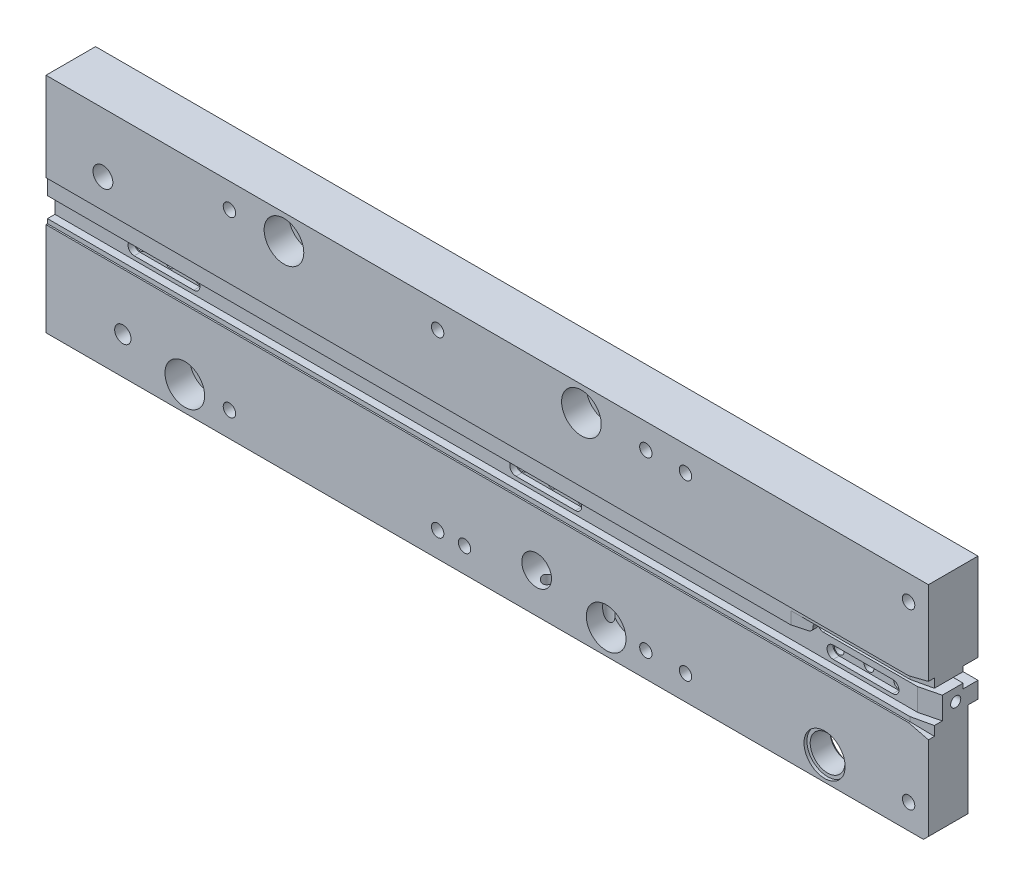
from build123d import *
from OCP.BRepFilletAPI import BRepFilletAPI_MakeChamfer

# Parameters (mm, degrees)
SKETCH1_W                                         = 350
SKETCH1_H                                         = 45
BOSS_EXTRUDE1_DEPTH                               = 10
CUT_EXTRUDE2_DEPTH                                = 0.3
CUT_EXTRUDE3_DEPTH                                = 1.8
CUT_EXTRUDE4_DEPTH                                = 177.72365433070925
CUT_EXTRUDE5_DEPTH                                = 3
CHAMFER1_SIZE                                     = 0.9
CHAMFER1_SIZE2                                    = 4
SKETCH7_W                                         = 55
SKETCH7_H                                         = 7.6
CUT_EXTRUDE6_DEPTH                                = 46.000000000000014
CUT_EXTRUDE7_DEPTH                                = 177.72365433070925
SKETCH9_W                                         = 49.99999999999999
SKETCH9_H                                         = 45
CUT_EXTRUDE8_DEPTH                                = 1.5
SKETCH10_R                                        = 2.249999999999996
SKETCH10_R_2                                      = 2.250000000000001
CUT_EXTRUDE9_DEPTH                                = 177.72365433070925
SKETCH11_R                                        = 4.000000000000006
SKETCH11_R_2                                      = 4
CUT_EXTRUDE10_DEPTH                               = 5
CUT_EXTRUDE11_START                               = -2.5
SKETCH12_R                                        = 4.000000000000006
SKETCH12_R_2                                      = 4.000000000000001
CUT_EXTRUDE11_DEPTH                               = 2.5
HOLE_SIZE_PER_HEX_BOLT_GRADE_C_TYPE_1_D           = 3.5
HOLE_SIZE_PER_HEX_BOLT_GRADE_C_TYPE_1_CBORE_D     = 6
HOLE_SIZE_PER_HEX_BOLT_GRADE_C_TYPE_1_CBORE_DEPTH = 5
SKETCH15_R                                        = 3.499999999999994
CUT_EXTRUDE12_DEPTH                               = 17.000000000000004
SKETCH19_W                                        = 24
SKETCH19_H                                        = 0.5000000000000346
CUT_EXTRUDE13_DEPTH                               = 6.999999999999998
CHAMFER2_SIZE                                     = 1
CHAMFER2_SIZE2                                    = 4
CHAMFER3_SIZE                                     = 4
CHAMFER3_SIZE2                                    = 1
CHAMFER4_SIZE                                     = 4
CHAMFER4_SIZE2                                    = 0.5
CUT_EXTRUDE14_REACH                               = 178.894
FILLET1_R                                         = 1
FILLET6_R                                         = 1
CUT_EXTRUDE15_DEPTH                               = 20
M3_TAPPED_HOLE2_D                                 = 2.5
M3_TAPPED_HOLE2_DEPTH                             = 7.5
M3_TAPPED_HOLE2_TIP                               = 0.7510757737844503
SKETCH30_R                                        = 3.999999999999999
SKETCH30_R_2                                      = 4.000000000000005
CUT_EXTRUDE20_DEPTH                               = 5
SKETCH31_R                                        = 2.2500000000000027
SKETCH31_R_2                                      = 2.2499999999999987
SKETCH31_R_3                                      = 2.2499999999999964
CUT_EXTRUDE21_DEPTH                               = 25.000000000000007
SKETCH32_W                                        = 54.999999999999986
SKETCH32_H                                        = 3
CUT_EXTRUDE22_DEPTH                               = 8
SKETCH33_R                                        = 3.9999999999999925
SKETCH33_R_2                                      = 4.000000000000005
CUT_EXTRUDE23_DEPTH                               = 5
SKETCH34_R                                        = 2.2500000000000093
SKETCH34_R_2                                      = 2.2499999999999964
CUT_EXTRUDE24_DEPTH                               = 19.000000000000004
SKETCH35_W                                        = 8
SKETCH35_H                                        = 8.000000000000007
CUT_EXTRUDE25_DEPTH                               = 5
M4_TAPPED_HOLE2_D                                 = 3.3
M4_TAPPED_HOLE2_DEPTH                             = 10.1
M4_TAPPED_HOLE2_TIP                               = 0.9914200213954745
SKETCH37_R                                        = 1.9999999999999996
CUT_EXTRUDE26_DEPTH                               = 6
CHAMFER5_SIZE                                     = 0.5
CHAMFER5_SIZE2                                    = 5
CHAMFER6_SIZE                                     = 5
CHAMFER6_SIZE2                                    = 0.5
FILLET8_R                                         = 1
M3_TAPPED_HOLE3_D                                 = 2.5
M3_TAPPED_HOLE3_DEPTH                             = 7.5
M3_TAPPED_HOLE3_TIP                               = 0.7510757737844503
CUT_EXTRUDE28_DEPTH                               = 3
SKETCH45_R                                        = 0.9999999999999983
SKETCH45_R_2                                      = 1.0000000000000016
CUT_EXTRUDE29_DEPTH                               = 5
SKETCH46_R                                        = 1.0000000000000002
CUT_EXTRUDE30_DEPTH                               = 50
SKETCH48_R                                        = 1.0000000000000016
SKETCH48_R_2                                      = 0.9999999999999983
CUT_EXTRUDE32_DEPTH                               = 177.72365433070925
CUT_EXTRUDE33_DEPTH                               = 2.5
SKETCH50_W                                        = 70.00000000000001
SKETCH50_H                                        = 26.641464115410763
CUT_EXTRUDE34_DEPTH                               = 60.00000000000003
SKETCH52_R                                        = 2.4999999999999796
CUT_EXTRUDE35_DEPTH                               = 10
M2_5_TAPPED_HOLE1_AT_2_COUNT                      = 2
M2_5_TAPPED_HOLE1_AT_2_PITCH                      = 8
SKETCH59_R                                        = 1.9999999999999967
CUT_EXTRUDE36_DEPTH                               = 5.5
FILLET9_R                                         = 3
FILLET10_R                                        = 1.5
CUT_EXTRUDE38_DEPTH                               = 96.00000000000003
CUT_EXTRUDE39_DEPTH                               = 2.8
SKETCH63_R                                        = 4.1499999999999835
CUT_EXTRUDE40_DEPTH                               = 0.6
SKETCH64_R                                        = 4.1499999999999835
CUT_EXTRUDE41_DEPTH                               = 0.6
FILLET11_R                                        = 1.5
M2_5_TAPPED_HOLE2_D                               = 2.05
M2_5_TAPPED_HOLE2_DEPTH                           = 5
M2_5_TAPPED_HOLE2_TIP                             = 0.6158821345032492
CHAMFER7_SIZE                                     = 1
BOSS_EXTRUDE2_DEPTH                               = 5.2


with BuildPart() as part:
    # Sketch1 → Boss-Extrude1 (new body)
    with BuildSketch(Plane.XY):
        Rectangle(SKETCH1_W, SKETCH1_H)
    extrude(amount=BOSS_EXTRUDE1_DEPTH)

    # Sketch3 → Cut-Extrude2 (cut)
    with BuildSketch(Plane.XY.offset(10)):
        Polygon((-175.00000000000003, 4.599999999999915), (174.99999999999997, 4.6), (174.99999999999997, -3.599999999999999), (-175.00000000000003, -3.599999999999999), align=None)
    extrude(amount=-CUT_EXTRUDE2_DEPTH, mode=Mode.SUBTRACT)

    # Sketch4 → Cut-Extrude3 (cut)
    with BuildSketch(Plane.XY.offset(10)):
        Polygon((174.99999999999997, 1.2999999999999654), (-175.00000000000003, 1.299999999999922), (-175.00000000000003, -2.7000000000000774), (174.99999999999997, -2.700000000000035), align=None)
    extrude(amount=-CUT_EXTRUDE3_DEPTH, mode=Mode.SUBTRACT)

    # Sketch5 → Cut-Extrude4 (cut, through all)
    with BuildSketch(Plane.XY.offset(10)):
        Polygon((150.99999999999997, 3.799999999999994), (174.99999999999997, 3.8), (174.99999999999997, 1.8), (150.99999999999997, 1.8), align=None)
    extrude(amount=-CUT_EXTRUDE4_DEPTH, mode=Mode.SUBTRACT)

    # Sketch6 → Cut-Extrude5 (cut)
    with BuildSketch(Plane(origin=(0, 0, 0), x_dir=(-1, 0, 0), z_dir=(0, 0, -1))):
        Polygon((-139.99999999999997, 0.8000000000000004), (-174.99999999999997, 0.7999999999999965), (-174.99999999999997, 4.799999999999997), (-139.99999999999997, 4.800000000000001), align=None)
    extrude(amount=-CUT_EXTRUDE5_DEPTH, mode=Mode.SUBTRACT)

    # Chamfer1: one chamfer whose edges measure the first distance from different faces: ONE call of the kernel's chamfer builder (chamfer() names one face for all edges)
    chamfer1_edges_1 = [part.edges().sort_by_distance(p)[0] for p in [
        (174.99999999999997, -3.1500000000000172, 9.7),
        (174.99999999999997, 1.5499999999999825, 9.7),
    ]]
    chamfer1_side_1 = [part.faces().sort_by_distance(p)[0] for p in [
        (174.99999999999997, -10.81544022721405, 4.909385489284791),
    ]]
    chamfer1_edges_2 = [part.edges().sort_by_distance(p)[0] for p in [
        (174.99999999999997, 4.199999999999999, 9.7),
    ]]
    chamfer1_side_2 = [part.faces().sort_by_distance(p)[0] for p in [
        (174.99999999999997, 13.306171092729647, 5.050805398345668),
    ]]
    chamfer1 = BRepFilletAPI_MakeChamfer(part.part.solid().wrapped)
    for e in chamfer1_edges_1:
        chamfer1.Add(CHAMFER1_SIZE, CHAMFER1_SIZE2, e.wrapped, chamfer1_side_1[0].wrapped)  # the first distance lies on this face
    for e in chamfer1_edges_2:
        chamfer1.Add(CHAMFER1_SIZE, CHAMFER1_SIZE2, e.wrapped, chamfer1_side_2[0].wrapped)  # the first distance lies on this face
    add(Compound.cast(chamfer1.Shape()), mode=Mode.REPLACE)

    # Sketch7 → Cut-Extrude6 (cut)
    with BuildSketch(Plane.XY.offset(10)):
        with Locations((-113, 0.49999999999998157)):
            Rectangle(SKETCH7_W, SKETCH7_H)
    extrude(amount=-CUT_EXTRUDE6_DEPTH, mode=Mode.SUBTRACT)

    # Sketch8 → Cut-Extrude7 (cut, through all)
    with BuildSketch(Plane.XY.offset(10)):
        Polygon((-63.00000000000003, 9.5), (-13.000000000000032, 9.5), (-13.000000000000028, -8.499999999999998), (-63.00000000000003, -8.499999999999998), align=None)
    extrude(amount=-CUT_EXTRUDE7_DEPTH, mode=Mode.SUBTRACT)

    # Sketch9 → Cut-Extrude8 (cut)
    with BuildSketch(Plane.XY.offset(10)):
        with Locations((-38.000000000000036, 0)):
            Rectangle(SKETCH9_W, SKETCH9_H)
    extrude(amount=-CUT_EXTRUDE8_DEPTH, mode=Mode.SUBTRACT)

    # Sketch10 → Cut-Extrude9 (cut, through all)
    with BuildSketch(Plane.XY.offset(10)):
        with Locations((-69, 11.49999999999999)):
            Circle(SKETCH10_R)
        with Locations((-69.00000000000001, -10.500000000000007)):
            Circle(SKETCH10_R)
        with Locations((-7.000000000000017, -10.500000000000018)):
            Circle(SKETCH10_R_2)
        with Locations((-7.00000000000001, 11.499999999999979)):
            Circle(SKETCH10_R_2)
    extrude(amount=-CUT_EXTRUDE9_DEPTH, mode=Mode.SUBTRACT)

    # Sketch11 → Cut-Extrude10 (cut)
    with BuildSketch(Plane.XY.offset(10)):
        with Locations((-69, 11.49999999999999)):
            Circle(SKETCH11_R)
        with Locations((-69.00000000000001, -10.500000000000007)):
            Circle(SKETCH11_R)
        with Locations((-7.000000000000017, -10.500000000000018)):
            Circle(SKETCH11_R_2)
        with Locations((-7.00000000000001, 11.499999999999979)):
            Circle(SKETCH11_R_2)
    extrude(amount=-CUT_EXTRUDE10_DEPTH, mode=Mode.SUBTRACT)

    # Sketch12 → Cut-Extrude11 (cut)
    with BuildSketch(Plane(origin=(0, 0, 0), x_dir=(-1, 0, 0), z_dir=(0, 0, -1)).offset(CUT_EXTRUDE11_START)):
        with Locations(Location((69, 11.49999999999999, 0), (0, 0, 180))):
            Circle(SKETCH12_R)
        with Locations(Location((7.000000000000017, -10.500000000000018, 0), (0, 0, 180))):
            Circle(SKETCH12_R_2)
    extrude(amount=CUT_EXTRUDE11_DEPTH, mode=Mode.SUBTRACT)

    # Hole size per hex bolt grade C type 1 (through all)
    with Locations(Plane(origin=(95.97, -14.5, 10), x_dir=(1, 0, 0), z_dir=(0, 0, 1))):
        with Locations((0, 0)):
            CounterBoreHole(HOLE_SIZE_PER_HEX_BOLT_GRADE_C_TYPE_1_D / 2, HOLE_SIZE_PER_HEX_BOLT_GRADE_C_TYPE_1_CBORE_D / 2, HOLE_SIZE_PER_HEX_BOLT_GRADE_C_TYPE_1_CBORE_DEPTH)

    # Sketch15 → Cut-Extrude12 (cut)
    with BuildSketch(Plane.XY.offset(10)):
        with Locations((154.04999999999995, -17.669999999999998)):
            Circle(SKETCH15_R)
    extrude(amount=-CUT_EXTRUDE12_DEPTH, mode=Mode.SUBTRACT)

    # Sketch19 → Cut-Extrude13 (cut)
    with BuildSketch(Plane.XY.offset(8.200000000000001)):
        with Locations((162.99999999999997, 1.5499999999999827)):
            Rectangle(SKETCH19_W, SKETCH19_H)
    extrude(amount=CUT_EXTRUDE13_DEPTH, mode=Mode.SUBTRACT)

    # Chamfer2: one chamfer whose edges measure the first distance from different faces: ONE call of the kernel's chamfer builder (chamfer() names one face for all edges)
    chamfer2_edges_1 = [part.edges().sort_by_distance(p)[0] for p in [
        (174.99999999999997, -0.4500000000000173, 8.2),
    ]]
    chamfer2_side_1 = [part.faces().sort_by_distance(p)[0] for p in [
        (174.99999999999997, -10.882518845853916, 4.88102417468157),
    ]]
    chamfer2_edges_2 = [part.edges().sort_by_distance(p)[0] for p in [
        (174.99999999999997, 4.6, 9.399999999999999),
    ]]
    chamfer2_side_2 = [part.faces().sort_by_distance(p)[0] for p in [
        (174.99999999999997, 13.341990821678323, 5.034287587412589),
    ]]
    chamfer2 = BRepFilletAPI_MakeChamfer(part.part.solid().wrapped)
    for e in chamfer2_edges_1:
        chamfer2.Add(CHAMFER2_SIZE, CHAMFER2_SIZE2, e.wrapped, chamfer2_side_1[0].wrapped)  # the first distance lies on this face
    for e in chamfer2_edges_2:
        chamfer2.Add(CHAMFER2_SIZE, CHAMFER2_SIZE2, e.wrapped, chamfer2_side_2[0].wrapped)  # the first distance lies on this face
    add(Compound.cast(chamfer2.Shape()), mode=Mode.REPLACE)

    # Chamfer3
    chamfer3_edges = [part.edges().sort_by_distance(p)[0] for p in [
        (174.99999999999997, -3.599999999999999, 9.399999999999999),
    ]]
    chamfer3_side = [part.faces().sort_by_distance(p)[0] for p in [
        (83.86597938144327, -3.599999999999999, 9.836082474226805),
    ]]
    chamfer(chamfer3_edges, length=CHAMFER3_SIZE, length2=CHAMFER3_SIZE2, reference=chamfer3_side[0])

    # Chamfer4
    chamfer4_edges = [part.edges().sort_by_distance(p)[0] for p in [
        (150.99999999999997, 1.2999999999999654, 8.95),
    ]]
    chamfer4_side = [part.faces().sort_by_distance(p)[0] for p in [
        (68.99999999999997, 1.2999999999999523, 8.95),
    ]]
    chamfer(chamfer4_edges, length=CHAMFER4_SIZE, length2=CHAMFER4_SIZE2, reference=chamfer4_side[0])

    # Cut-Extrude14: up to this face of the body (flat: up to its plane)
    cut_extrude14_end = Plane(part.part.faces().sort_by_distance((162.879245283, 3.8, 6.315471698))[0])
    # Sketch21 → Cut-Extrude14 (cut, up to the picked face)
    with BuildSketch(Plane.XZ.offset(-1.2999999999999439), mode=Mode.PRIVATE) as cut_extrude14_sk1:
        Polygon((146.99999999999986, 9.700000000000001), (151.5522483304892, 9.700000000000001), (151.5522483304892, 9.2), align=None)
    cut_extrude14_tool1 = split(extrude(cut_extrude14_sk1.sketch, amount=-CUT_EXTRUDE14_REACH, mode=Mode.PRIVATE), bisect_by=cut_extrude14_end, keep=Keep.BOTH, mode=Mode.PRIVATE)
    add(cut_extrude14_tool1.solids().sort_by(Axis((150.034832, 1.3, 9.533333), (-1.2e-16, 1, 0)))[0], mode=Mode.SUBTRACT)

    # Fillet1
    fillet1_edges = [part.edges().sort_by_distance(p)[0] for p in [
        (150.99999999999997, 3.799999999999994, 6.1303283284652155),
    ]]
    fillet(fillet1_edges, radius=FILLET1_R)

    # Fillet6
    fillet6_edges = [part.edges().sort_by_distance(p)[0] for p in [
        (150.99999999999997, 1.7999999999999625, 8.730328328465212),
    ]]
    fillet(fillet6_edges, radius=FILLET6_R)

    # Sketch22 → Cut-Extrude15 (cut)
    with BuildSketch(Plane.XZ.offset(22.5)):
        Polygon((174.99999999999997, 0), (139.99999999999997, -4.29e-15), (139.99999999999997, 1.9999999999999958), (174.99999999999997, 2), align=None)
    extrude(amount=-CUT_EXTRUDE15_DEPTH, mode=Mode.SUBTRACT)

    # M3 Tapped Hole2
    with Locations(Plane.XY.offset(10)):
        with Locations((34, -17.5), (34, 17.5), (76, -17.5), (76, 17.5), (118, -17.5), (118, 17.5), (126, 17.5), (126, -17.5), (171, -17.5), (171, 17.5)):
            Hole(M3_TAPPED_HOLE2_D / 2, depth=M3_TAPPED_HOLE2_DEPTH)
            with Locations((0, 0, -(M3_TAPPED_HOLE2_DEPTH + M3_TAPPED_HOLE2_TIP / 2))):  # 118° drill point
                Cone(0, M3_TAPPED_HOLE2_D / 2, M3_TAPPED_HOLE2_TIP, mode=Mode.SUBTRACT)

    # Sketch30 → Cut-Extrude20 (cut)
    with BuildSketch(Plane.XY.offset(10)):
        with Locations((24.99999999999994, -17.499999999999996)):
            Circle(SKETCH30_R)
        with Locations((109.99999999999994, -17.499999999999996)):
            Circle(SKETCH30_R_2)
        with Locations((104.99999999999996, 17.499999999999996)):
            Circle(SKETCH30_R_2)
        with Locations((44.99999999999996, 17.499999999999996)):
            Circle(SKETCH30_R_2)
    extrude(amount=-CUT_EXTRUDE20_DEPTH, mode=Mode.SUBTRACT)

    # Sketch31 → Cut-Extrude21 (cut)
    with BuildSketch(Plane.XY.offset(10)):
        with Locations((44.99999999999996, 17.499999999999996)):
            Circle(SKETCH31_R)
        with Locations((24.99999999999994, -17.499999999999996)):
            Circle(SKETCH31_R_2)
        with Locations((109.99999999999994, -17.499999999999996)):
            Circle(SKETCH31_R_3)
        with Locations((104.99999999999996, 17.499999999999996)):
            Circle(SKETCH31_R_3)
    extrude(amount=-CUT_EXTRUDE21_DEPTH, mode=Mode.SUBTRACT)

    # Sketch32 → Cut-Extrude22 (cut)
    with BuildSketch(Plane.XZ.offset(22.5)):
        with Locations((-105.5, 1.5)):
            Rectangle(SKETCH32_W, SKETCH32_H)
    extrude(amount=-CUT_EXTRUDE22_DEPTH, mode=Mode.SUBTRACT)

    # Sketch33 → Cut-Extrude23 (cut)
    with BuildSketch(Plane.XY.offset(10)):
        with Locations((-160.00000000000003, 17.499999999999996)):
            Circle(SKETCH33_R)
        with Locations((-95.00000000000003, 17.499999999999996)):
            Circle(SKETCH33_R_2)
        with Locations((-160.00000000000003, -17.499999999999996)):
            Circle(SKETCH33_R)
    extrude(amount=-CUT_EXTRUDE23_DEPTH, mode=Mode.SUBTRACT)

    # Sketch34 → Cut-Extrude24 (cut)
    with BuildSketch(Plane.XY.offset(10)):
        with Locations((-160.00000000000003, 17.499999999999996)):
            Circle(SKETCH34_R)
        with Locations((-160.00000000000003, -17.499999999999996)):
            Circle(SKETCH34_R)
        with Locations((-95.00000000000003, 17.499999999999996)):
            Circle(SKETCH34_R_2)
    extrude(amount=-CUT_EXTRUDE24_DEPTH, mode=Mode.SUBTRACT)

    # Sketch35 → Cut-Extrude25 (cut)
    with BuildSketch(Plane.XY.offset(10)):
        with Locations((-160.00000000000003, 21.5)):
            Rectangle(SKETCH35_W, SKETCH35_H)
        with Locations((-95.00000000000003, 21.5)):
            Rectangle(SKETCH35_W, SKETCH35_H)
        with Locations((-160.00000000000003, -21.5)):
            Rectangle(SKETCH35_W, SKETCH35_H)
    extrude(amount=-CUT_EXTRUDE25_DEPTH, mode=Mode.SUBTRACT)

    # M4 Tapped Hole2
    with Locations(Plane(origin=(12.5, -15, 10), x_dir=(1, 0, 0), z_dir=(0, 0, 1))):
        with Locations((0, 0)):
            Hole(M4_TAPPED_HOLE2_D / 2, depth=M4_TAPPED_HOLE2_DEPTH)
            with Locations((0, 0, -(M4_TAPPED_HOLE2_DEPTH + M4_TAPPED_HOLE2_TIP / 2))):  # 118° drill point
                Cone(0, M4_TAPPED_HOLE2_D / 2, M4_TAPPED_HOLE2_TIP, mode=Mode.SUBTRACT)

    # Sketch37 → Cut-Extrude26 (cut)
    with BuildSketch(Plane.XY.offset(10)):
        with Locations((8.47999999999996, 10.500000000000002)):
            Circle(SKETCH37_R)
    extrude(amount=-CUT_EXTRUDE26_DEPTH, mode=Mode.SUBTRACT)

    # Chamfer5: one chamfer whose edges measure the first distance from different faces: ONE call of the kernel's chamfer builder (chamfer() names one face for all edges)
    chamfer5_edges_1 = [part.edges().sort_by_distance(p)[0] for p in [
        (-140.5, -2.7000000000000735, 8.95),
        (-140.5, 1.299999999999926, 8.950000000000001),
    ]]
    chamfer5_side_1 = [part.faces().sort_by_distance(p)[0] for p in [
        (-140.5, 0.6063201417601755, 4.486739515652685),
    ]]
    chamfer5_edges_2 = [part.edges().sort_by_distance(p)[0] for p in [
        (-63.00000000000003, -3.5999999999999996, 9.85),
        (-63.00000000000003, -2.7000000000000637, 8.95),
        (-63.00000000000002, 1.2999999999999359, 8.95),
        (-63.00000000000003, 4.599999999999943, 9.85),
    ]]
    chamfer5_side_2 = [part.faces().sort_by_distance(p)[0] for p in [
        (-63.00000000000003, 0.3747877758913459, 5.643718166383701),
    ]]
    chamfer5 = BRepFilletAPI_MakeChamfer(part.part.solid().wrapped)
    for e in chamfer5_edges_1:
        chamfer5.Add(CHAMFER5_SIZE, CHAMFER5_SIZE2, e.wrapped, chamfer5_side_1[0].wrapped)  # the first distance lies on this face
    for e in chamfer5_edges_2:
        chamfer5.Add(CHAMFER5_SIZE, CHAMFER5_SIZE2, e.wrapped, chamfer5_side_2[0].wrapped)  # the first distance lies on this face
    add(Compound.cast(chamfer5.Shape()), mode=Mode.REPLACE)

    # Chamfer6: one chamfer whose edges measure the first distance from different faces: ONE call of the kernel's chamfer builder (chamfer() names one face for all edges)
    chamfer6_edges_1 = [part.edges().sort_by_distance(p)[0] for p in [
        (-63.00000000000003, -3.6500000000000314, 9.7),
        (-140.5, -3.2500000000000453, 9.7),
    ]]
    chamfer6_side_1 = [part.faces().sort_by_distance(p)[0] for p in [
        (-76.75000000000001, -2.812008749658295, 9.7),
    ]]
    chamfer6_edges_2 = [part.edges().sort_by_distance(p)[0] for p in [
        (-63.00000000000003, 3.449999999999939, 9.7),
        (-140.5, 3.0499999999999527, 9.7),
    ]]
    chamfer6_side_2 = [part.faces().sort_by_distance(p)[0] for p in [
        (-160.25, 2.420644457443943, 9.7),
    ]]
    chamfer6 = BRepFilletAPI_MakeChamfer(part.part.solid().wrapped)
    for e in chamfer6_edges_1:
        chamfer6.Add(CHAMFER6_SIZE, CHAMFER6_SIZE2, e.wrapped, chamfer6_side_1[0].wrapped)  # the first distance lies on this face
    for e in chamfer6_edges_2:
        chamfer6.Add(CHAMFER6_SIZE, CHAMFER6_SIZE2, e.wrapped, chamfer6_side_2[0].wrapped)  # the first distance lies on this face
    add(Compound.cast(chamfer6.Shape()), mode=Mode.REPLACE)

    # Fillet8
    fillet8_edges = [part.edges().sort_by_distance(p)[0] for p in [
        (-85.5, -3.3000000000000185, 4.85),
        (-85.5, 4.299999999999981, 4.85),
        (-140.5, -3.3000000000000185, 4.6),
        (-140.5, 4.299999999999981, 4.6),
    ]]
    fillet(fillet8_edges, radius=FILLET8_R)

    # M3 Tapped Hole3
    with Locations(Plane.XY.offset(8.5)):
        with Locations((-57, -16), (-19, -16), (-19, 17), (-57, 17)):
            Hole(M3_TAPPED_HOLE3_D / 2, depth=M3_TAPPED_HOLE3_DEPTH)
            with Locations((0, 0, -(M3_TAPPED_HOLE3_DEPTH + M3_TAPPED_HOLE3_TIP / 2))):  # 118° drill point
                Cone(0, M3_TAPPED_HOLE3_D / 2, M3_TAPPED_HOLE3_TIP, mode=Mode.SUBTRACT)

    # Sketch44 → Cut-Extrude28 (cut)
    with BuildSketch(Plane.XY.offset(10)):
        with BuildLine():
            Line((165.99999999999994, -1.9500000000000404), (153.99999999999994, -1.9500000000000417))
            ThreePointArc((153.99999999999994, -1.9500000000000417), (152.74999999999994, -0.7000000000000418), (153.99999999999994, 0.5499999999999583))
            Line((153.99999999999994, 0.5499999999999583), (165.99999999999994, 0.5499999999999601))
            ThreePointArc((165.99999999999994, 0.5499999999999601), (167.24999999999994, -0.7000000000000408), (165.99999999999994, -1.9500000000000404))
        make_face()
        with BuildLine():
            Line((101.99999999999997, -1.950000000000045), (89.99999999999997, -1.9500000000000468))
            ThreePointArc((89.99999999999997, -1.9500000000000468), (88.74999999999997, -0.700000000000047), (89.99999999999997, 0.5499999999999524))
            Line((89.99999999999997, 0.5499999999999524), (101.99999999999997, 0.5499999999999537))
            ThreePointArc((101.99999999999997, 0.5499999999999537), (103.24999999999997, -0.7000000000000444), (101.99999999999997, -1.950000000000045))
        make_face()
        with BuildLine():
            Line((12.999999999999966, 0.5499999999999424), (24.999999999999968, 0.5499999999999424))
            ThreePointArc((24.999999999999968, 0.5499999999999424), (26.249999999999964, -0.7000000000000582), (24.999999999999968, -1.950000000000056))
            Line((24.999999999999968, -1.950000000000056), (12.999999999999966, -1.950000000000056))
            ThreePointArc((12.999999999999966, -1.950000000000056), (11.749999999999966, -0.700000000000057), (12.999999999999966, 0.5499999999999424))
        make_face()
    extrude(amount=-CUT_EXTRUDE28_DEPTH, mode=Mode.SUBTRACT)

    # Sketch45 → Cut-Extrude29 (cut)
    with BuildSketch(Plane.XY.offset(10)):
        with Locations((165.99999999999994, -0.7000000000000408)):
            Circle(SKETCH45_R)
        with Locations((153.99999999999994, -0.7000000000000419)):
            Circle(SKETCH45_R)
        with Locations((101.99999999999997, -0.7000000000000444)):
            Circle(SKETCH45_R)
        with Locations((89.99999999999997, -0.7000000000000471)):
            Circle(SKETCH45_R)
        with Locations((24.999999999999968, -0.7000000000000582)):
            Circle(SKETCH45_R_2)
        with Locations((12.999999999999966, -0.7000000000000571)):
            Circle(SKETCH45_R_2)
        with Locations((159.99999999999994, -0.7000000000000413)):
            Circle(SKETCH45_R)
        with Locations((96.0000000000018, -0.6999999999974267)):
            Circle(SKETCH45_R)
        with Locations((18.999999999988503, -0.6999999999974267)):
            Circle(SKETCH45_R_2)
    extrude(amount=-CUT_EXTRUDE29_DEPTH, mode=Mode.SUBTRACT)

    # Sketch46 → Cut-Extrude30 (cut)
    with BuildSketch(Plane(origin=(174.99999999999997, 0, 0), x_dir=(0, 0, -1), z_dir=(1, 0, 0))):
        with Locations((-4.5, -0.6999999999999993)):
            Circle(SKETCH46_R)
    extrude(amount=-CUT_EXTRUDE30_DEPTH, mode=Mode.SUBTRACT)

    # Sketch48 → Cut-Extrude32 (cut, through all)
    with BuildSketch(Plane.XY.offset(10)):
        with Locations((12.999999999999966, -0.7000000000000571)):
            Circle(SKETCH48_R)
        with Locations((18.999999999988503, -0.6999999999974267)):
            Circle(SKETCH48_R)
        with Locations((24.999999999999968, -0.7000000000000582)):
            Circle(SKETCH48_R)
        with Locations((101.99999999999997, -0.7000000000000444)):
            Circle(SKETCH48_R_2)
        with Locations((96.0000000000018, -0.6999999999974267)):
            Circle(SKETCH48_R_2)
        with Locations((89.99999999999997, -0.7000000000000471)):
            Circle(SKETCH48_R_2)
    extrude(amount=-CUT_EXTRUDE32_DEPTH, mode=Mode.SUBTRACT)

    # Sketch49 → Cut-Extrude33 (cut)
    with BuildSketch(Plane(origin=(0, 0, 0), x_dir=(-1, 0, 0), z_dir=(0, 0, -1))):
        with BuildLine():
            Line((-103.50000000000182, 1.3000000000025718), (-88.50000000000182, 1.3000000000025707))
            ThreePointArc((-88.50000000000182, 1.3000000000025707), (-86.5000000000018, -0.6999999999974215), (-88.5000000000018, -2.699999999997429))
            Line((-88.5000000000018, -2.699999999997429), (-103.50000000000182, -2.699999999997429))
            ThreePointArc((-103.50000000000182, -2.699999999997429), (-105.50000000000182, -0.6999999999974283), (-103.50000000000182, 1.3000000000025718))
        make_face()
        with BuildLine():
            Line((-26.499999999988507, 1.3000000000025913), (-11.499999999988495, 1.3000000000025913))
            ThreePointArc((-11.499999999988495, 1.3000000000025913), (-9.499999999988496, -0.6999999999974087), (-11.499999999988495, -2.6999999999974076))
            Line((-11.499999999988495, -2.6999999999974076), (-26.499999999988507, -2.6999999999974076))
            ThreePointArc((-26.499999999988507, -2.6999999999974076), (-28.499999999988507, -0.6999999999974085), (-26.499999999988507, 1.3000000000025913))
        make_face()
    extrude(amount=-CUT_EXTRUDE33_DEPTH, mode=Mode.SUBTRACT)

    # Sketch50 → Cut-Extrude34 (cut)
    with BuildSketch(Plane(origin=(0, 22.5, 0), x_dir=(1, 0, 0), z_dir=(0, 1, 0))):
        with Locations((-38.000000000000036, 0)):
            Rectangle(SKETCH50_W, SKETCH50_H)
    extrude(amount=-CUT_EXTRUDE34_DEPTH, mode=Mode.SUBTRACT)


with BuildPart() as cut_extrude34_piece_1:
    # of the separate pieces the step leaves, piece 1, a body of its own (cut_extrude34_pieces)
    add(part.part.solids().sort_by_distance((-3, 22.5, 0))[0])

    # Sketch51 → M3 Tapped Hole4 (revolve, cut)
    with BuildSketch(Plane(origin=(95.96999999999996, -22.5, 7.5), x_dir=(0, 0, -1), z_dir=(1, 0, 0))):
        Polygon((0, 0), (-2.02e-15, 8.25107577378445), (1.2499999999999976, 7.5), (1.2499999999999987, -5e-17), align=None)
    revolve(axis=Axis((95.96999999999996, -28.84999999999999, 7.5), (0, 1, 0)), mode=Mode.SUBTRACT)

    # Sketch52 → Cut-Extrude35 (cut)
    with BuildSketch(Plane.XZ.offset(22.5)):
        with Locations(Location((81.41999999999996, 3.999999999999949, 0), (0, 0, 270))):
            Circle(SKETCH52_R)
    extrude(amount=-CUT_EXTRUDE35_DEPTH, mode=Mode.SUBTRACT)

    # Sketch53 → M3 Tapped Hole5 (revolve, cut)
    with BuildSketch(Plane(origin=(81.41999999999996, -17.499999999999996, 10), x_dir=(0, -1, 0), z_dir=(1, 0, 0))):
        Polygon((0, 0), (-2.02e-15, 8.251075773784452), (1.2499999999999871, 7.499999999999993), (1.249999999999989, -1.4e-15), align=None)
    revolve(axis=Axis((81.41999999999996, -17.499999999999996, 16.34999999999999), (0, 0, -1)), mode=Mode.SUBTRACT)

    # Sketch55 → M2.5 Tapped Hole1 (revolve, cut)
    with BuildSketch(Plane(origin=(113.99999999999996, -22.5, 5.7), x_dir=(0, 0, -1), z_dir=(1, 0, 0))):
        Polygon((0, 0), (-1.71e-15, 6.965882134503248), (1.0249999999999984, 6.35), (1.024999999999999, -3e-17), align=None)
    m2_5_tapped_hole1 = revolve(axis=Axis((113.99999999999996, -28.84999999999999, 5.7), (0, 1, 0)), mode=Mode.SUBTRACT)

    # M2.5 Tapped Hole1 at 2: M2.5 Tapped Hole1 ×2
    with Locations(*[(-i * M2_5_TAPPED_HOLE1_AT_2_PITCH, 0, 0) for i in range(1, M2_5_TAPPED_HOLE1_AT_2_COUNT)]):
        add(m2_5_tapped_hole1, mode=Mode.SUBTRACT)

    # Sketch59 → Cut-Extrude36 (cut)
    with BuildSketch(Plane(origin=(0, 0, 0), x_dir=(-1, 0, 0), z_dir=(0, 0, -1))):
        with Locations((-124.99999999999996, -0.6999999999999993)):
            Circle(SKETCH59_R)
    extrude(amount=-CUT_EXTRUDE36_DEPTH, mode=Mode.SUBTRACT)

    # Fillet9
    fillet9_edges = [cut_extrude34_piece_1.edges().sort_by_distance(p)[0] for p in [
        (139.99999999999997, -2.5, 0.9999999999999957),
    ]]
    fillet(fillet9_edges, radius=FILLET9_R)

    # Fillet10
    fillet10_edges = [cut_extrude34_piece_1.edges().sort_by_distance(p)[0] for p in [
        (139.99999999999997, 4.800000000000001, 1.5),
        (139.99999999999997, 0.8000000000000004, 1.5),
    ]]
    fillet(fillet10_edges, radius=FILLET10_R)

    # Sketch62 → Cut-Extrude39 (cut)
    with BuildSketch(Plane(origin=(-2.5e-16, 0, 1.9999999999999785), x_dir=(-1, 0, -1.2e-16), z_dir=(1.2e-16, 0, -1))):
        Polygon((-164.04999999999998, -30.002737548386204), (-144.04999999999995, -30.0027375483862), (-144.04999999999995, -10), (-164.04999999999998, -10.000000000000002), align=None)
    extrude(amount=-CUT_EXTRUDE39_DEPTH, mode=Mode.SUBTRACT)

    # Sketch63 → Cut-Extrude40 (cut)
    with BuildSketch(Plane.XY.offset(10)):
        with Locations((154.04999999999995, -17.669999999999998)):
            Circle(SKETCH63_R)
    extrude(amount=-CUT_EXTRUDE40_DEPTH, mode=Mode.SUBTRACT)

    # Sketch64 → Cut-Extrude41 (cut)
    with BuildSketch(Plane(origin=(-6.2e-16, 0, 4.799999999999978), x_dir=(-1, 0, -1.3e-16), z_dir=(1.3e-16, 0, -1))):
        with Locations(Location((-154.04999999999995, -17.669999999999998, 0), (0, 0, 180))):
            Circle(SKETCH64_R)
    extrude(amount=-CUT_EXTRUDE41_DEPTH, mode=Mode.SUBTRACT)

    # Fillet11
    fillet11_edges = [cut_extrude34_piece_1.edges().sort_by_distance(p)[0] for p in [
        (144.04999999999995, -10, 3.399999999999996),
        (164.04999999999998, -10.000000000000002, 3.3999999999999986),
    ]]
    fillet(fillet11_edges, radius=FILLET11_R)

    # M2.5 Tapped Hole2
    with Locations(Plane(origin=(175, -0.7, 4.5), x_dir=(0, 0, 1), z_dir=(1, 0, 0))):
        with Locations((0, 0)):
            Hole(M2_5_TAPPED_HOLE2_D / 2, depth=M2_5_TAPPED_HOLE2_DEPTH)
            with Locations((0, 0, -(M2_5_TAPPED_HOLE2_DEPTH + M2_5_TAPPED_HOLE2_TIP / 2))):  # 118° drill point
                Cone(0, M2_5_TAPPED_HOLE2_D / 2, M2_5_TAPPED_HOLE2_TIP, mode=Mode.SUBTRACT)

    # Chamfer7
    chamfer7_edges = [cut_extrude34_piece_1.edges().sort_by_distance(p)[0] for p in [
        (174.99999999999997, -22.5, 6),
    ]]
    chamfer(chamfer7_edges, length=CHAMFER7_SIZE)

    # Sketch69 → Boss-Extrude2 (add)
    with BuildSketch(Plane.XY.offset(8.200000000000001)):
        with BuildLine():
            Line((151.99999999999997, 1.7999999999999963), (151.99999999999997, 1.6330437825662754))
            Line((151.99999999999997, 1.6330437825662754), (150.99999999999997, 1.6330437825662754))
            Line((150.99999999999997, 1.6330437825662754), (150.99999999999997, 2.7999999999999945))
            ThreePointArc((150.99999999999997, 2.7999999999999945), (151.29289321881342, 2.092893218813447), (151.99999999999997, 1.7999999999999963))
        make_face()
    extrude(amount=-BOSS_EXTRUDE2_DEPTH)


with BuildPart() as cut_extrude34_piece_2:
    # of the separate pieces the step leaves, piece 2, a body of its own (cut_extrude34_pieces)
    add(part.part.solids().sort_by_distance((-85.5, 3.3, 9.7))[0])

    # Sketch61 → Cut-Extrude38 (cut)
    with BuildSketch(Plane.XZ.offset(22.5)):
        Polygon((-3.00000000000003, 10), (-183.00000000000003, 9.999999999999977), (-183.00000000000003, -10.000000000000023), (-3.000000000000028, -10), align=None)
    extrude(amount=-CUT_EXTRUDE38_DEPTH, mode=Mode.SUBTRACT)


solid = cut_extrude34_piece_1.part
